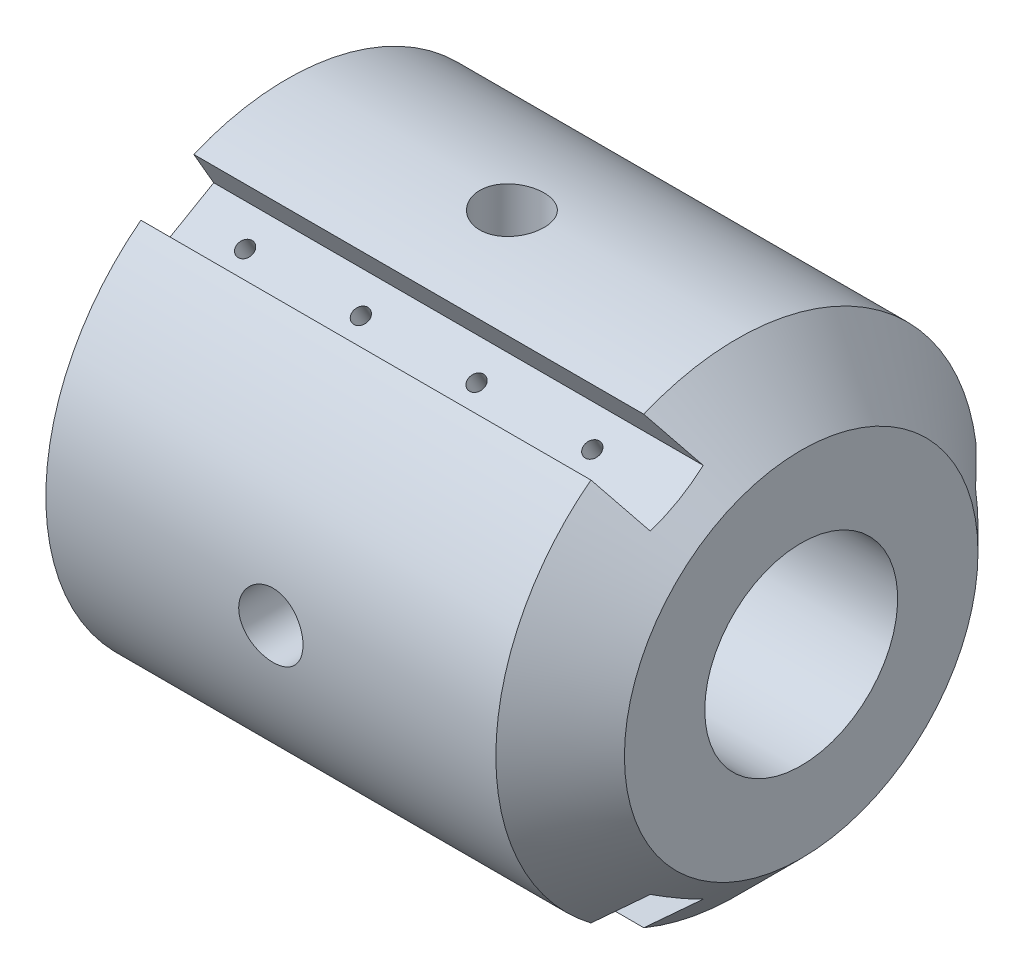
SolidWorks part; units mm, degrees
ref_plane "Front" through (0, 0, 0) normal (0, 0, 1) x (1, 0, 0)
ref_plane "Top" through (0, 0, 0) normal (0, 1, 0) x (1, 0, 0)
ref_plane "Right" through (0, 0, 0) normal (1, 0, 0) x (0, 0, -1)
sketch "Sketch1" plane through (0, 0, 0) normal (0, 0, 1) x (1, 0, 0)
  line L0 (0, 0) -> (80.8839, 0) construction
  line L1 (0, 15) -> (0, 37.5)
  line L2 (0, 37.5) -> (80, 37.5)
  line L3 (80, 37.5) -> (80, 15)
  line L4 (80, 15) -> (0, 15)
  dimension "D1" = 30
  dimension "D2" = 75
  dimension "D3" = 80
revolve "Revolve1" add sketch "Sketch1" angle 360 about L0
chamfer "Chamfer1" distance 10 angle 45 1 edges at (80, 0, 37.5)
sketch "Sketch2" plane through (0, 0, 0) normal (0, 0, 1) x (1, 0, 0)
  line L0 (0, 0) -> (80, 0) construction
  line L1 (80, -27.5) -> (80, 27.5) construction
  line L3 (0, 37.5) -> (0, -37.5) construction
  circle A1 centre (35, 0) radius 5
  dimension "D1" = 35
  dimension "D2" = 10
extrude "Cut-Extrude1" cut sketch "Sketch2" along normal through all from offset 22.5
hole_wizard "M5 Tapped Hole1" positions "Sketch4" profile "Sketch3" tap size "M5" standard "GB"
sketch "Sketch4" plane through (-1.8297, 1.0496, 22.5) normal (0, 0, 1) x (1, 0, 0)
  circle A1 centre (36.8297, -1.0496) radius 5 construction
  point P1 (36.8297, -1.0496)
sketch "Sketch3" plane through (35, 0, 22.5) normal (1, 0, 0) x (0, -1, 0)
  line L0 (0, 0) -> (0, 13.6618)
  line L1 (0, 13.6618) -> (2.1, 12.4)
  line L2 (2.1, 12.4) -> (2.1, 0)
  line L5 (2.1, 0) -> (0, 0)
  line L10 (0, 13.6618) -> (-2.1, 12.4) construction
  line L11 (0, -6.35) -> (0, 107.95) construction
  dimension "螺纹孔钻头直径" = 4.2
  dimension "螺纹孔钻头深度" = 12.4
  dimension "导头角度" = 118
cosmetic thread "Cosmetic Thread2" parameters "D1"=7.6477, "D2"=5
pattern_circular "CirPattern1" count 2 over 90 about axis through (0, 0, 0) along (-1, 0, 0) of "Cut-Extrude1", "M5 Tapped Hole1"
sketch "Sketch5" plane through (80, 0, 0) normal (1, 0, 0) x (0, 0, -1)
  line L0 (0, 0) -> (70.709, 0) construction
  line L1 (31, 4.75) -> (44, 4.75)
  line L2 (31, 4.75) -> (31, -4.75)
  line L3 (31, -4.75) -> (44, -4.75)
  line L4 (44, 4.75) -> (44, -4.75)
  line L5 (31, 4.75) -> (44, -4.75) construction
  line L6 (31, -4.75) -> (44, 4.75) construction
  circle A0 centre (0, 0) radius 37.5 construction
  point P0 (37.5, 0)
  dimension "D1" = 9.5
  dimension "D2" = 31
extrude "Cut-Extrude2" cut sketch "Sketch5" against normal through all
hole_wizard "M3 Tapped Hole1" positions "Sketch7" profile "Sketch6" tap size "M3" standard "Gb"
sketch "Sketch7" plane through (0, 0, -31) normal (0, 0, -1) x (-1, 0, 0)
  line L0 (0, 0) -> (-88.3599, 0) construction
  line L2 (0, -37.5) -> (0, 37.5) construction
  point P0 (-45, 0)
  point P2 (-63, 0)
  point P4 (-27, 0)
  point P6 (-9, 0)
  dimension "D1" = 18
  dimension "D2" = 18
  dimension "D3" = 18
  dimension "D4" = 9
sketch "Sketch6" plane through (45, 0, -31) normal (1, 0, 0) x (0, 1, 0)
  line L0 (0, 0) -> (0, 8.2511)
  line L1 (0, 8.2511) -> (1.25, 7.5)
  line L2 (1.25, 7.5) -> (1.25, 0)
  line L5 (1.25, 0) -> (0, 0)
  line L10 (0, 8.2511) -> (-1.25, 7.5) construction
  line L11 (0, -6.35) -> (0, 107.95) construction
  dimension "螺纹孔钻头直径" = 2.5
  dimension "螺纹孔钻头深度" = 7.5
  dimension "导头角度" = 118
cosmetic thread "Cosmetic Thread3" parameters "D1"=6, "D2"=3
cosmetic thread "Cosmetic Thread4" parameters "D1"=6, "D2"=3
cosmetic thread "Cosmetic Thread5" parameters "D1"=6, "D2"=3
cosmetic thread "Cosmetic Thread6" parameters "D1"=6, "D2"=3
pattern_circular "CirPattern2" count 3 every 120 about axis through (0, 0, 0) along (1, 0, 0) of "Cut-Extrude2", "M3 Tapped Hole1"
